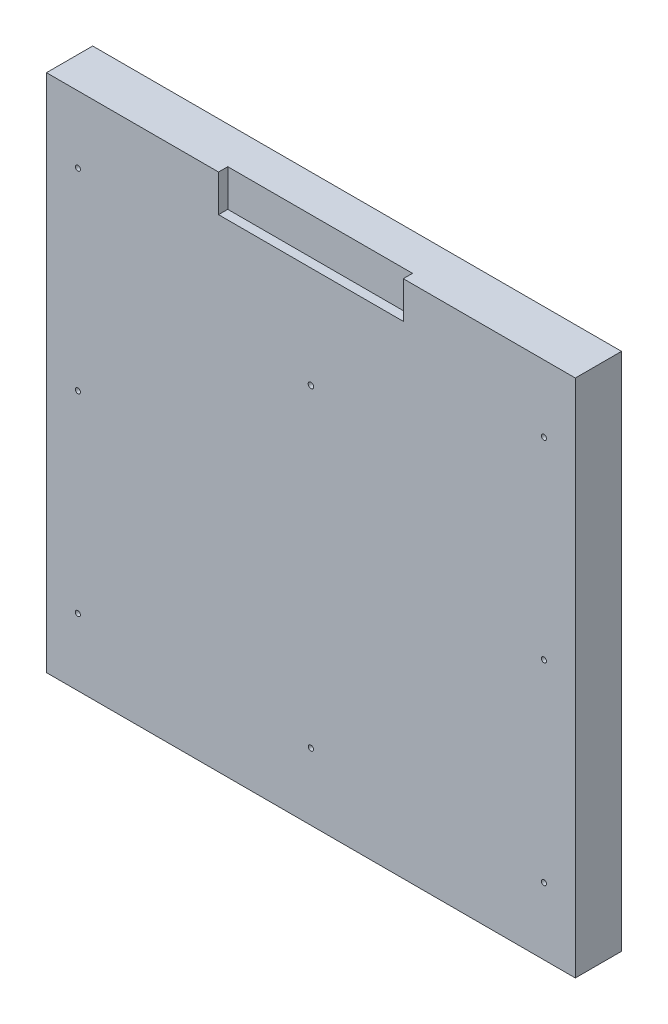
SolidWorks part; units mm, degrees
material "普通碳钢"
ref_plane "前视基准面" through (0, 0, 0) normal (0, 0, 1) x (1, 0, 0)
ref_plane "上视基准面" through (0, 0, 0) normal (0, 1, 0) x (1, 0, 0)
ref_plane "右视基准面" through (0, 0, 0) normal (1, 0, 0) x (0, 0, -1)
sketch "草图1" plane through (0, 0, 0) normal (0, 0, 1) x (1, 0, 0)
  line L1 (-572.5, 562.5) -> (572.5, 562.5)
  line L2 (-572.5, 562.5) -> (-572.5, -562.5)
  line L3 (-572.5, -562.5) -> (572.5, -562.5)
  line L4 (572.5, 562.5) -> (572.5, -562.5)
  line L5 (-572.5, 562.5) -> (572.5, -562.5) construction
  line L6 (-572.5, -562.5) -> (572.5, 562.5) construction
  point P0 (0, 0)
extrude "凸台-拉伸1" add sketch "草图1" along normal blind 100
sketch "草图2" plane through (0, 0, 100) normal (0, 0, 1) x (1, 0, 0)
  line L0 (572.5, 562.5) -> (-572.5, 562.5) construction
  line L1 (-200, 642.5) -> (200, 642.5)
  line L2 (-200, 642.5) -> (-200, 482.5)
  line L3 (-200, 482.5) -> (200, 482.5)
  line L4 (200, 642.5) -> (200, 482.5)
  line L5 (-200, 642.5) -> (200, 482.5) construction
  line L6 (-200, 482.5) -> (200, 642.5) construction
  point P0 (0, 562.5)
extrude "切除-拉伸1" cut sketch "草图2" against normal blind 20
sketch "草图3" plane through (0, 0, 100) normal (0, 0, 1) x (1, 0, 0)
  line L0 (200, 562.5) -> (-200, 562.5) construction
  circle A0 centre (0, 262.5) radius 6
  dimension "D1" = 12
  dimension "D2" = 300
sketch "草图4" plane through (0, 0, 100) normal (0, 0, 1) x (1, 0, 0)
  line L0 (-200, 562.5) -> (-572.5, 562.5) construction
  line L1 (-572.5, 562.5) -> (-572.5, -562.5) construction
  line L2 (0, 0) -> (0, 309.7933) construction
  line L3 (0, 0) -> (177.4665, 0) construction
  line L4 (-572.5, -562.5) -> (572.5, -562.5) construction
  line L5 (-504.5, -417.5) -> (504.5, -417.5) construction
  line L6 (-504.5, 139.1667) -> (-504.5, -139.1667) construction
  circle A0 centre (-504.5, 417.5) radius 5.5
  circle A1 centre (-504.5, 139.1667) radius 5.5 construction
  circle A2 centre (-504.5, -139.1667) radius 5.5 construction
  circle A3 centre (-504.5, -417.5) radius 5.5
  circle A4 centre (504.5, -417.5) radius 5.5
  circle A5 centre (504.5, -139.1667) radius 5.5 construction
  circle A6 centre (504.5, 139.1667) radius 5.5 construction
  circle A7 centre (504.5, 417.5) radius 5.5
  circle A8 centre (0, -417.5) radius 5.5
  circle A9 centre (-504.5, 0) radius 5.5
  circle A10 centre (504.5, 0) radius 5.5
  dimension "D1" = 145
  dimension "D2" = 68
  dimension "D3" = 11
  dimension "D5" = 145
  dimension "D6" = 11
  dimension "D4" = 4
extrude "切除-拉伸2" cut sketch "草图4" against normal through all both and the other way through all
extrude "切除-拉伸3" cut sketch "草图3" against normal through all both and the other way through all
equation "\"A\" = 1245"
equation "\"B\" = 1245"
equation "\"CH\" = 2220"
equation "\"OP\" = 800"
equation "\"OPH\" = 2100"
equation "\"QB\" = 50"
equation "\"DK\" = 40"
equation "\"WCOP\" = 0"
equation "\"HCOP\" = 4"
equation "\"FJ\" = 2"
equation "\"DH\" = 16"
equation "\"LG\" = 1"
equation "\"DD\" = 3"
equation "\"C\" = 590"
equation "\"PX\" = -50"
equation "\"LZ\" = 350"
equation "\"LJ\" = 1258"
equation "\"LLK\" = 310"
equation "\"FS\" = 0"
equation "\"D2@草图1\" = \"吊顶深度\""
equation "\"D1@草图1\"= \"吊顶宽度\""
equation "\"D2@草图2\"=IF(\"FJ\" =1,140,80.00mm)"
equation "\"CW\"= \"A\" - 60"
equation "\"吊顶宽度\"= \"CW\" - 40"
equation "\"CD\"= \"B\" - 30 - \"QB\""
equation "\"吊顶深度\"= \"CD\" - 40"
